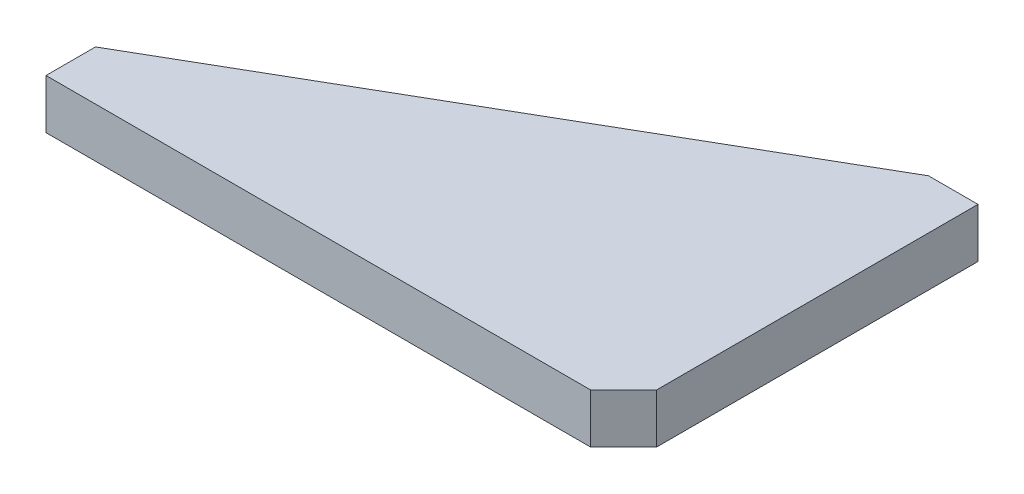
from build123d import *

# Parameters (mm, degrees)
EXTRUDE_1_DEPTH = 30


with BuildPart() as part:
    # 草图1 → 凸台-拉伸1 (new body)
    with BuildSketch(Plane(origin=(0, 0, 0), x_dir=(1, 0, 0), z_dir=(0, 1, 0))):
        Polygon((0, 0), (-30, 0), (-350, -184.752086141), (-350, -214.752086141), (-20, -214.752086141), (0, -194.752086141), align=None)
    extrude(amount=EXTRUDE_1_DEPTH)


solid = part.part
